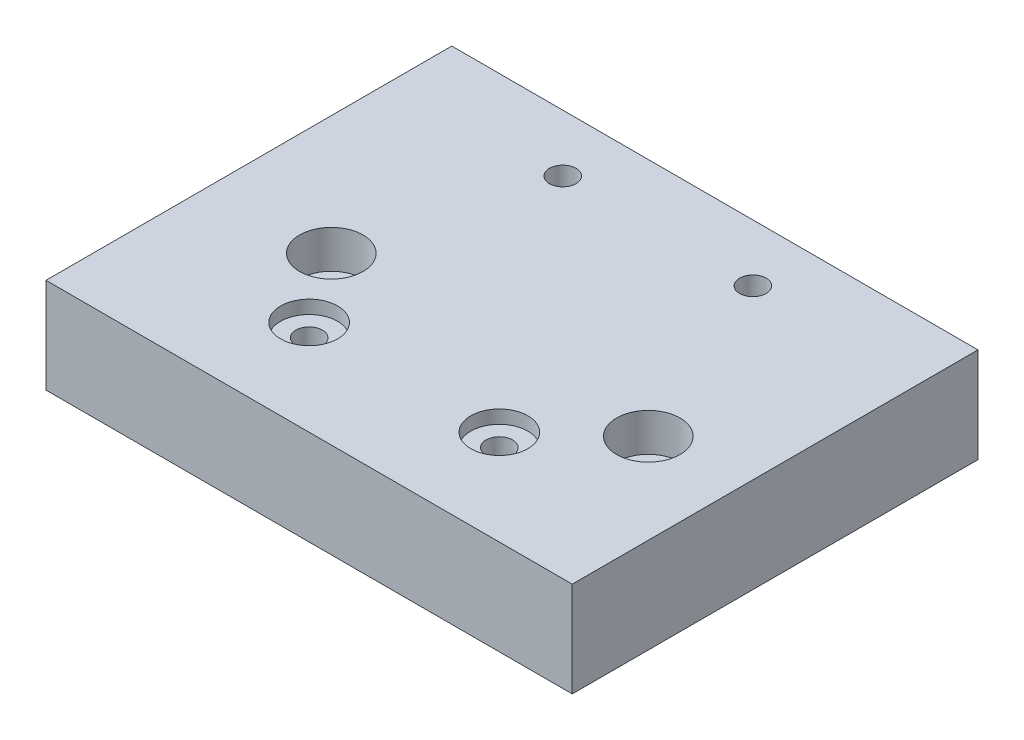
from build123d import *

# Parameters (mm, degrees)
SKETCH1_W                                            = 83
SKETCH1_H                                            = 15
BOSS_EXTRUDE1_DEPTH                                  = 64
HOLE_SIZE_PER_SOCKET_HEAD_CAP_SCREW_TYPE_D           = 5.5
HOLE_SIZE_PER_SOCKET_HEAD_CAP_SCREW_TYPE_CBORE_D     = 10
HOLE_SIZE_PER_SOCKET_HEAD_CAP_SCREW_TYPE_CBORE_DEPTH = 6
SKETCH5_R                                            = 3.5
CUT_EXTRUDE1_DEPTH                                   = 1.6
M5_TAPPED_HOLE1_D                                    = 4.2
SKETCH8_R                                            = 4.5
CUT_EXTRUDE2_DEPTH                                   = 2.1


with BuildPart() as part:
    # Sketch1 → Boss-Extrude1 (new body)
    with BuildSketch(Plane.XY):
        with Locations((41.5, 7.5)):
            Rectangle(SKETCH1_W, SKETCH1_H)
    extrude(amount=BOSS_EXTRUDE1_DEPTH)

    # Hole size per socket head cap screw type 1 (through all)
    with Locations(Plane(origin=(0, 15, 0), x_dir=(1, 0, 0), z_dir=(0, 1, 0))):
        with Locations((18.8, -37.8), (68.8, -37.8)):
            CounterBoreHole(HOLE_SIZE_PER_SOCKET_HEAD_CAP_SCREW_TYPE_D / 2, HOLE_SIZE_PER_SOCKET_HEAD_CAP_SCREW_TYPE_CBORE_D / 2, HOLE_SIZE_PER_SOCKET_HEAD_CAP_SCREW_TYPE_CBORE_DEPTH)

    # Sketch5 → Cut-Extrude1 (cut)
    with BuildSketch(Plane.XZ):
        with Locations(Location((18.8, 37.8, 0), (0, 0, 270))):
            Circle(SKETCH5_R)
        with Locations(Location((68.8, 37.8, 0), (0, 0, 270))):
            Circle(SKETCH5_R)
    extrude(amount=-CUT_EXTRUDE1_DEPTH, mode=Mode.SUBTRACT)

    # M5 Tapped Hole1 (through all)
    with Locations(Plane(origin=(0, 15, 0), x_dir=(1, 0, 0), z_dir=(0, 1, 0))):
        with Locations((56.5, -9), (26.5, -9), (26.5, -49), (56.5, -49)):
            Hole(M5_TAPPED_HOLE1_D / 2)

    # Sketch8 → Cut-Extrude2 (cut)
    with BuildSketch(Plane(origin=(0, 15, 0), x_dir=(1, 0, 0), z_dir=(0, 1, 0))):
        with Locations(Location((26.5, -49, 0), (0, 0, 270))):
            Circle(SKETCH8_R)
        with Locations(Location((56.5, -49, 0), (0, 0, 270))):
            Circle(SKETCH8_R)
    extrude(amount=-CUT_EXTRUDE2_DEPTH, mode=Mode.SUBTRACT)


solid = part.part
